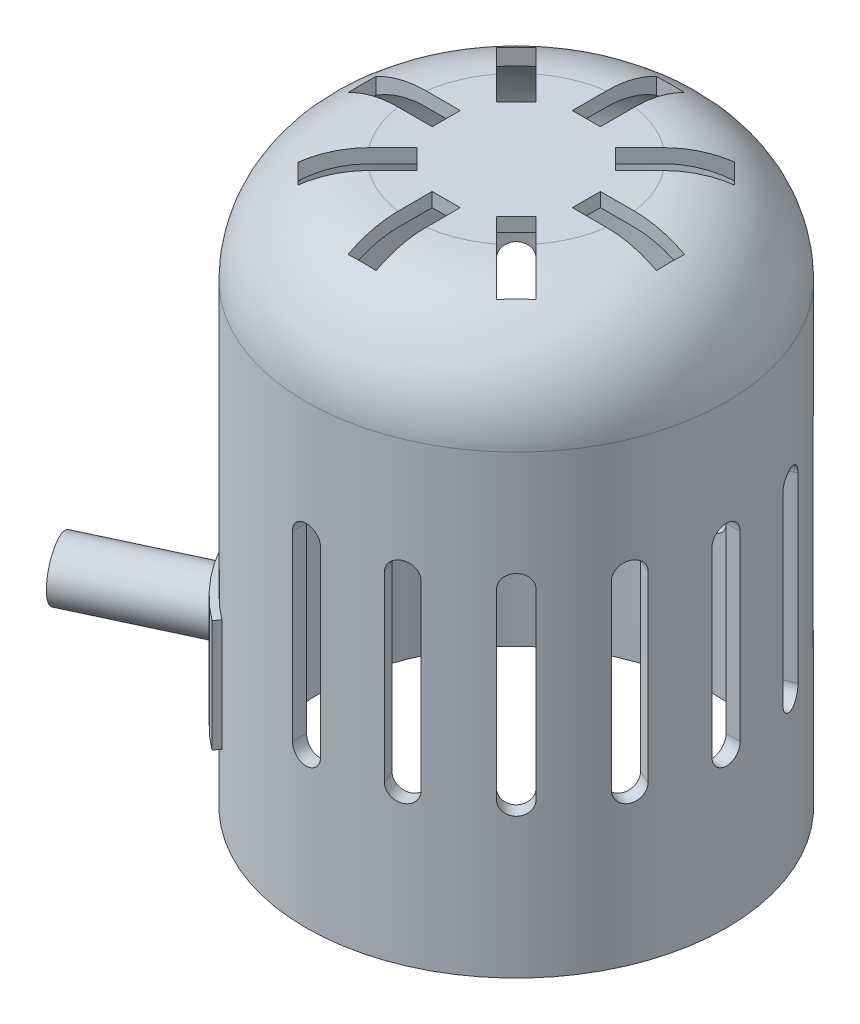
SolidWorks part; units mm, degrees
ref_plane "Front Plane" through (0, 0, 0) normal (0, 0, 1) x (1, 0, 0)
ref_plane "Top Plane" through (0, 0, 0) normal (0, 1, 0) x (1, 0, 0)
ref_plane "Right Plane" through (0, 0, 0) normal (1, 0, 0) x (0, 0, -1)
sketch "Sketch1" plane through (0, 0, 0) normal (0, 1, 0) x (1, 0, 0)
  circle A0 centre (0, 0) radius 30
  dimension "D1" = 60
extrude "Boss-Extrude3" add sketch "Sketch1" along normal blind 80
fillet "Fillet3" radius 15 1 edges at (0, 80, 30)
shell "Shell3" thickness 2
ref_plane "Plane1" through (0, 78, 0) normal (0, 1, 0) x (1, 0, 0)
sketch "Sketch3" plane through (0, 78, 0) normal (0, 1, 0) x (1, 0, 0)
  line L0 (-59.5888, 0) -> (64.74, 0) construction
  line L1 (0, 48.0465) -> (0, -52.4542) construction
  line L2 (14.1421, 16.9706) -> (16.9706, 14.1421)
  line L3 (-2, 22) -> (2, 22)
  line L4 (-2, 22) -> (-2, 10)
  line L5 (-2, 10) -> (2, 10)
  line L6 (2, 22) -> (2, 10)
  line L7 (-2, 22) -> (2, 10) construction
  line L8 (-2, 10) -> (2, 22) construction
  line L9 (14.1421, 16.9706) -> (5.6569, 8.4853)
  line L10 (5.6569, 8.4853) -> (8.4853, 5.6569)
  line L11 (16.9706, 14.1421) -> (8.4853, 5.6569)
  line L12 (22, 2) -> (22, -2)
  line L13 (22, 2) -> (10, 2)
  line L14 (10, 2) -> (10, -2)
  line L15 (22, -2) -> (10, -2)
  line L16 (16.9706, -14.1421) -> (14.1421, -16.9706)
  line L17 (16.9706, -14.1421) -> (8.4853, -5.6569)
  line L18 (8.4853, -5.6569) -> (5.6569, -8.4853)
  line L19 (14.1421, -16.9706) -> (5.6569, -8.4853)
  line L20 (2, -22) -> (-2, -22)
  line L21 (2, -22) -> (2, -10)
  line L22 (2, -10) -> (-2, -10)
  line L23 (-2, -22) -> (-2, -10)
  line L24 (-14.1421, -16.9706) -> (-16.9706, -14.1421)
  line L25 (-14.1421, -16.9706) -> (-5.6569, -8.4853)
  line L26 (-5.6569, -8.4853) -> (-8.4853, -5.6569)
  line L27 (-16.9706, -14.1421) -> (-8.4853, -5.6569)
  line L28 (-22, -2) -> (-22, 2)
  line L29 (-22, -2) -> (-10, -2)
  line L30 (-10, -2) -> (-10, 2)
  line L31 (-22, 2) -> (-10, 2)
  line L32 (-16.9706, 14.1421) -> (-14.1421, 16.9706)
  line L33 (-16.9706, 14.1421) -> (-8.4853, 5.6569)
  line L34 (-8.4853, 5.6569) -> (-5.6569, 8.4853)
  line L35 (-14.1421, 16.9706) -> (-5.6569, 8.4853)
  point P5 (0, 16)
  point P41 (0, 0)
  dimension "D1" = 12
  dimension "D2" = 4
  dimension "D3" = 10
  dimension "D4" = 8
extrude "Cut-Extrude4" cut sketch "Sketch3" against normal mid plane 20
sketch "Sketch4" plane through (0, 0, 0) normal (0, 0, 1) x (1, 0, 0)
  line L0 (0, 83.9135) -> (0, -8.064) construction
  line L1 (0, 48) -> (0, 22) construction
  line L2 (2, 48) -> (2, 22)
  line L3 (-2, 48) -> (-2, 22)
  arc A0 (2, 48) -> (-2, 48) centre (0, 48) ccw
  arc A1 (-2, 22) -> (2, 22) centre (0, 22) ccw
  point P5 (0, 35)
  dimension "D1" = 26
  dimension "D3" = 2
  dimension "D2" = 22
extrude "Cut-Extrude5" cut sketch "Sketch4" against normal blind 66
pattern_circular "CirPattern1" count 16 over 360 about axis through (0, 0, 0) along (0, 1, 0) skipping 3, 4, 5, 6, 7 of "Cut-Extrude5"
ref_plane "Plane3" through (0, 10, 0) normal (0, -1, 0) x (-1, 0, 0)
sketch "Sketch15" plane through (0, 10, 0) normal (0, -1, 0) x (-1, 0, 0)
  line L0 (29.9623, 1.5032) -> (30.9611, 1.5533)
  line L1 (18.0743, -23.9441) -> (18.6767, -24.7423)
  arc A0 (29.9623, 1.5032) -> (18.0743, -23.9441) centre (0, 0) cw
  circle A1 centre (0, 0) radius 30 construction
  arc A2 (30.9611, 1.5533) -> (18.6767, -24.7423) centre (0, 0) cw
  dimension "D1" = 1
extrude "Boss-Extrude4" add sketch "Sketch15" against normal blind 16
ref_plane "Plane4" through (-28.0955, 0, 13.1012) normal (-0.9063, 0, 0.4226) x (0, -1, 0)
sketch "Sketch16" plane through (-28.0955, 0, 13.1012) normal (-0.9063, 0, 0.4226) x (0, -1, 0)
  circle A0 centre (-17.5875, 0) radius 4
  dimension "D1" = 8
extrude "Boss-Extrude5" add sketch "Sketch16" along normal blind 18 separate body
